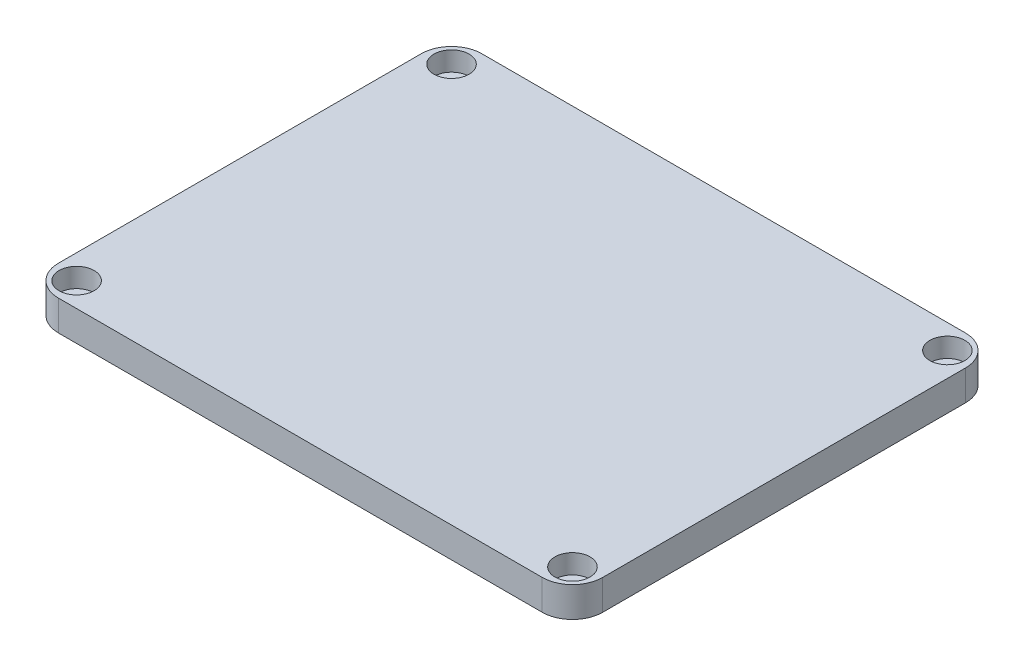
from build123d import *

# Parameters (mm, degrees)
SKETCH1_R           = 1.6
BOSS_EXTRUDE1_DEPTH = 5
SKETCH2_R           = 2.9
CUT_EXTRUDE1_DEPTH  = 3.2


with BuildPart() as part:
    # Sketch1 → Boss-Extrude1 (new body)
    with BuildSketch(Plane(origin=(0, 0, 0), x_dir=(1, 0, 0), z_dir=(0, 1, 0))):
        with BuildLine():
            Line((-40, -35), (40, -35))
            ThreePointArc((40, -35), (43.535533906, -33.535533906), (45, -30))
            Line((45, -30), (45, 30))
            ThreePointArc((45, 30), (43.535533906, 33.535533906), (40, 35))
            Line((40, 35), (-40, 35))
            ThreePointArc((-40, 35), (-43.535533906, 33.535533906), (-45, 30))
            Line((-45, 30), (-45, -30))
            ThreePointArc((-45, -30), (-43.535533906, -33.535533906), (-40, -35))
        make_face()
        with Locations(Location((-41, 31, 0), (0, 0, 270))):
            Circle(SKETCH1_R, mode=Mode.SUBTRACT)
        with Locations(Location((-41, -31, 0), (0, 0, 270))):
            Circle(SKETCH1_R, mode=Mode.SUBTRACT)
        with Locations(Location((41, -31, 0), (0, 0, 270))):
            Circle(SKETCH1_R, mode=Mode.SUBTRACT)
        with Locations(Location((41, 31, 0), (0, 0, 270))):
            Circle(SKETCH1_R, mode=Mode.SUBTRACT)
    extrude(amount=BOSS_EXTRUDE1_DEPTH)

    # Sketch2 → Cut-Extrude1 (cut)
    with BuildSketch(Plane(origin=(0, 5, 0), x_dir=(1, 0, 0), z_dir=(0, 1, 0))):
        with Locations(Location((41, 31, 0), (0, 0, 270))):
            Circle(SKETCH2_R)
        with Locations(Location((-41, 31, 0), (0, 0, 270))):
            Circle(SKETCH2_R)
        with Locations(Location((-41, -31, 0), (0, 0, 270))):
            Circle(SKETCH2_R)
        with Locations(Location((41, -31, 0), (0, 0, 270))):
            Circle(SKETCH2_R)
    extrude(amount=-CUT_EXTRUDE1_DEPTH, mode=Mode.SUBTRACT)


solid = part.part
